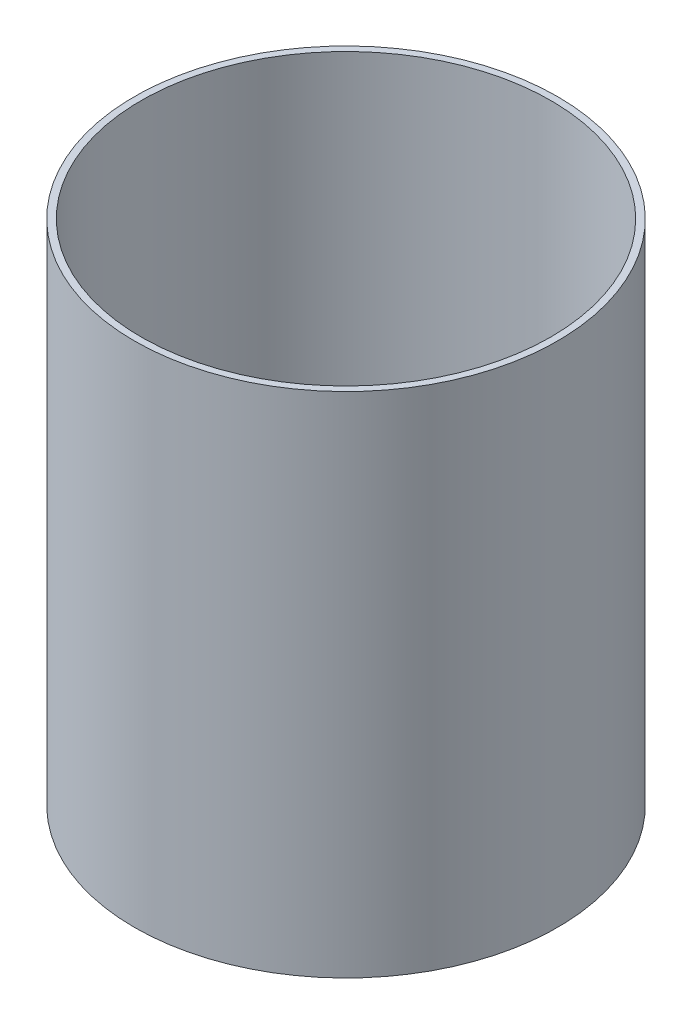
SolidWorks part; units mm, degrees
material "Q235"
ref_plane "前视基准面" through (0, 0, 0) normal (0, 0, 1) x (1, 0, 0)
ref_plane "上视基准面" through (0, 0, 0) normal (0, 1, 0) x (1, 0, 0)
ref_plane "右视基准面" through (0, 0, 0) normal (1, 0, 0) x (0, 0, -1)
sketch "草图1" plane through (0, 0, 0) normal (0, 1, 0) x (1, 0, 0)
  circle A0 centre (0, 0) radius 125
  dimension "D1" = 250
extrude "拉伸-薄壁1" add sketch "草图1" along normal blind 300 thin thin type one direction reverse wall 4
